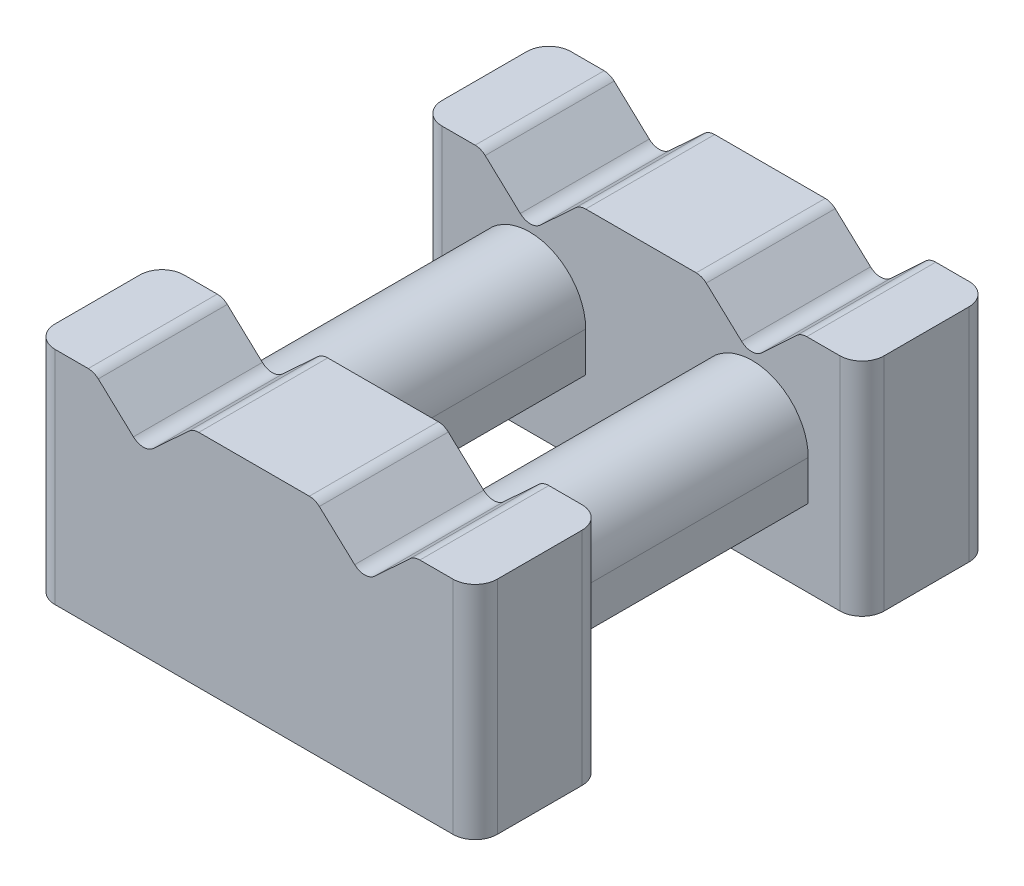
SolidWorks part; units mm, degrees
ref_plane "前视基准面" through (0, 0, 0) normal (0, 0, 1) x (1, 0, 0)
ref_plane "上视基准面" through (0, 0, 0) normal (0, 1, 0) x (1, 0, 0)
ref_plane "右视基准面" through (0, 0, 0) normal (1, 0, 0) x (0, 0, -1)
other "Configuration Table"
sketch "草图1" plane through (0, 0, 0) normal (0, 0, 1) x (1, 0, 0)
  line L0 (-3.7229, 4.8614) -> (2.2771, 4.8614)
  line L1 (2.2771, 4.8614) -> (2.2771, 1.8614)
  line L2 (-3.7229, 4.8614) -> (-3.7229, 1.8614)
  line L3 (-3.7229, 1.8614) -> (2.2771, 1.8614)
  dimension "D1" = 6
  dimension "D2" = 3
extrude "凸台-拉伸1" add sketch "草图1" along normal blind 1.75
sketch "草图2" plane through (0, 0, 0) normal (0, 0, -1) x (-1, 0, 0)
  line L4 (-2.2771, 4.8614) -> (3.7229, 4.8614) construction
  line L6 (0.7229, 4.8614) -> (0.7229, -49995.1386) construction
  line L10 (-0.0974, 2.9114) -> (-0.0271, 2.9114)
  line L13 (-1.5471, 2.9114) -> (-1.4568, 2.9114)
  line L26 (-1.5471, 3.4514) -> (-1.5471, 2.9114)
  line L27 (-0.0271, 3.4514) -> (-0.0271, 2.9114)
  line L28 (1.4729, 3.4514) -> (1.4729, 2.9114)
  line L29 (2.9929, 3.4514) -> (2.9929, 2.9114)
  line L30 (2.9929, 2.9114) -> (2.9026, 2.9114)
  line L31 (1.5432, 2.9114) -> (1.4729, 2.9114)
  line L32 (-2.2771, 1.8614) -> (-2.2771, 4.8614) construction
  line L33 (3.7229, 1.8614) -> (-2.2771, 1.8614) construction
  arc A10 (-1.4568, 2.9114) -> (-0.0974, 2.9114) centre (-0.7771, 3.2514) ccw
  arc A14 (-0.0271, 3.4514) -> (-1.5471, 3.4514) centre (-0.7871, 3.4514) ccw
  arc A17 (1.4729, 3.4514) -> (2.9929, 3.4514) centre (2.2329, 3.4514) cw
  arc A18 (2.9026, 2.9114) -> (1.5432, 2.9114) centre (2.2229, 3.2514) cw
  point P2 (-0.7771, 2.8614)
  point P12 (-0.7771, 2.4914)
  point P17 (0.7229, 4.8614)
  point P22 (2.2229, 3.3614)
  point P23 (2.2229, 2.8614)
  point P25 (-1.5471, 3.1814)
  point P28 (-0.7871, 4.2114)
  point P32 (-0.7771, 3.3614)
  dimension "D1" = 0.42
  dimension "D2" = 0.76
  dimension "D3" = 1.5
  dimension "D5" = 0.76
  dimension "D4" = 1.5
  dimension "D6" = 0.73
  dimension "D7" = 0.65
  dimension "D8" = 0.63
extrude "凸台-拉伸2" add sketch "草图2" along normal blind 3.5
ref_plane "基准面1" through (0, 0, -3.5) normal (0, 0, -1) x (-1, 0, 0)
fillet "圆角5" radius 0.3 1 edges at (2.2771, 3.3614, 1.75)
fillet "圆角6" radius 0.3 1 edges at (2.2771, 3.3614, 0)
fillet "圆角7" radius 0.3 1 edges at (-3.7229, 3.3614, 1.75)
fillet "圆角8" radius 0.3 1 edges at (-3.7229, 3.3614, 0)
sketch "草图6" plane through (0, 0, -3.5) normal (0, 0, -1) x (-1, 0, 0)
  line L0 (-2.2771, 4.8614) -> (3.7229, 4.8614)
  line L1 (3.7229, 4.8614) -> (3.7229, 1.8614)
  line L2 (3.7229, 1.8614) -> (-2.2771, 1.8614)
  line L3 (-2.2771, 1.8614) -> (-2.2771, 4.8614)
extrude "凸台-拉伸4" add sketch "草图6" along normal blind 1.75
fillet "圆角9" radius 0.3 1 edges at (2.2771, 3.3614, -5.25)
fillet "圆角10" radius 0.3 1 edges at (2.2771, 3.3614, -3.5)
fillet "圆角11" radius 0.3 1 edges at (-3.7229, 3.3614, -5.25)
fillet "圆角12" radius 0.3 1 edges at (-3.7229, 3.3614, -3.5)
sketch "草图7" plane through (0, 0, 1.75) normal (0, 0, 1) x (1, 0, 0)
  line L0 (-2.9729, 4.8614) -> (-1.4729, 4.8614)
  line L1 (-0.7229, 4.8614) -> (-0.7229, 50004.8614) construction
  line L2 (1.9771, 4.8614) -> (-3.4229, 4.8614) construction
  line L3 (0.1629, 4.8083) -> (0.6426, 4.3646)
  line L4 (1.3909, 4.8079) -> (0.9146, 4.365)
  line L5 (1.5271, 4.8614) -> (0.0271, 4.8614)
  line L10 (-2.8367, 4.8079) -> (-2.3603, 4.365)
  line L11 (-1.6087, 4.8083) -> (-2.0883, 4.3646)
  arc A4 (-2.8367, 4.8079) -> (-2.9729, 4.8614) centre (-2.9729, 4.6614) ccw
  arc A5 (-1.4729, 4.8614) -> (-1.6087, 4.8083) centre (-1.4729, 4.6614) ccw
  arc A6 (-2.3603, 4.365) -> (-2.0883, 4.3646) centre (-2.2242, 4.5114) ccw
  arc A7 (0.9146, 4.365) -> (0.6426, 4.3646) centre (0.7784, 4.5114) cw
  arc A8 (0.0271, 4.8614) -> (0.1629, 4.8083) centre (0.0271, 4.6614) cw
  arc A9 (1.3909, 4.8079) -> (1.5271, 4.8614) centre (1.5271, 4.6614) cw
  point P4 (-0.7229, 4.8614)
  dimension "D7" = 0.4
  dimension "D8" = 0.4
  dimension "D9" = 0.4
extrude "切除-拉伸1" cut sketch "草图7" against normal through all
